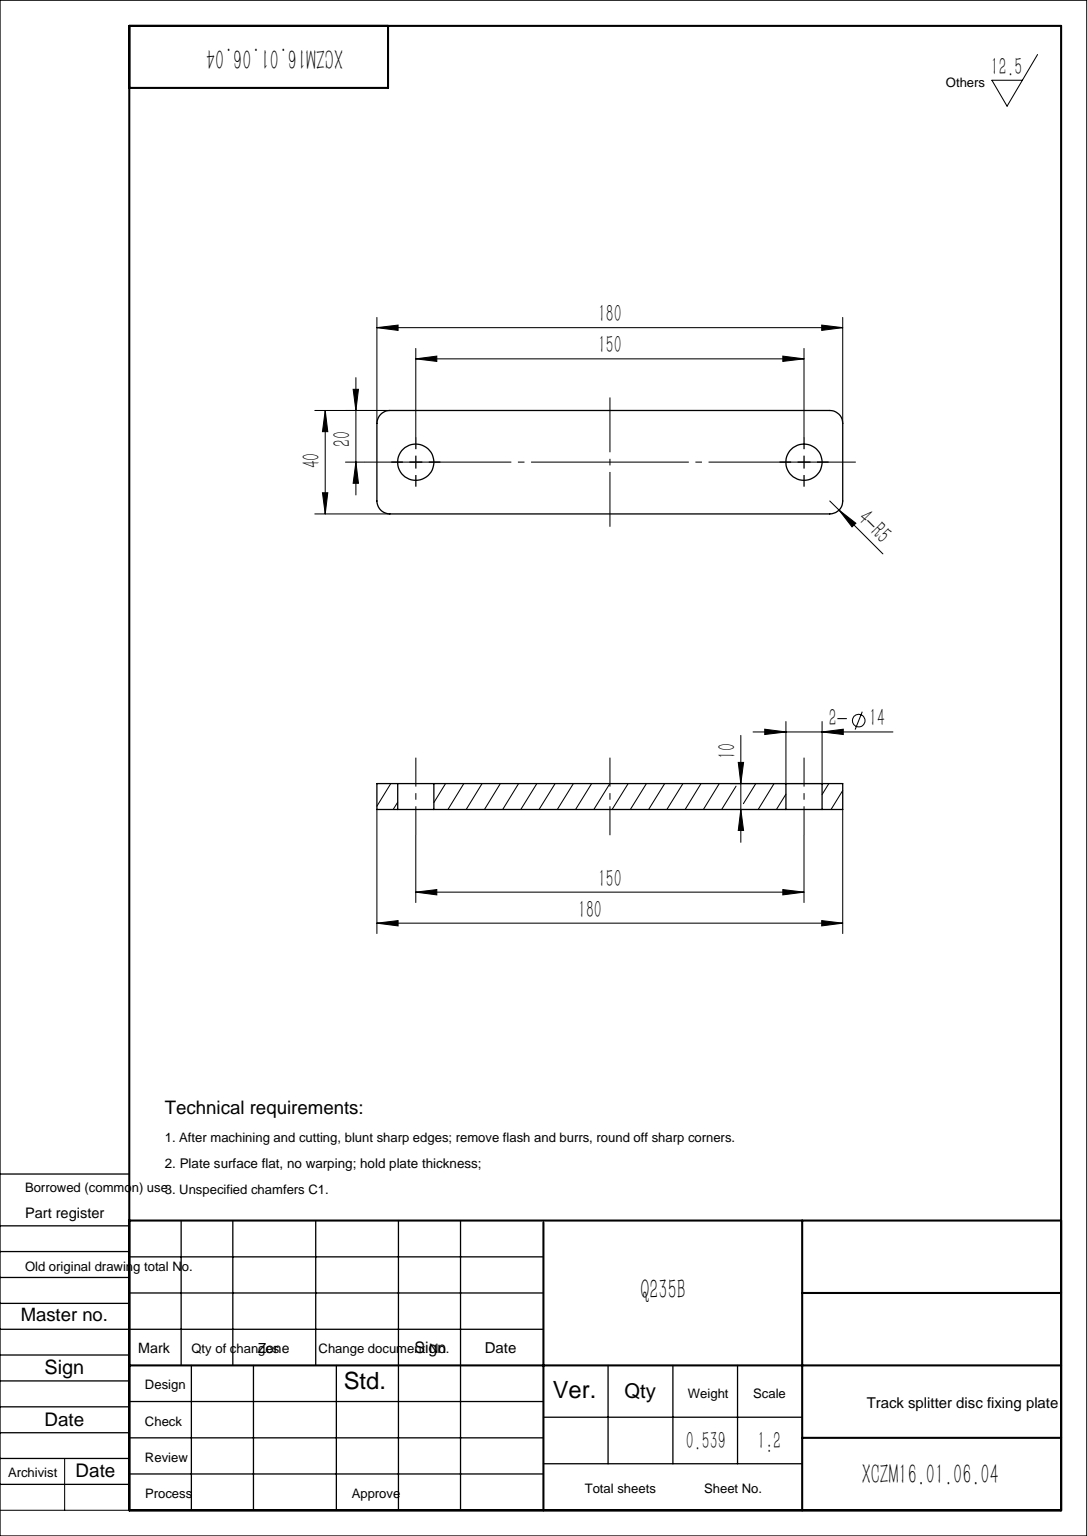
from build123d import *

# Parameters (mm, degrees)
SKETCH2_R           = 7
BOSS_EXTRUDE1_DEPTH = 10


with BuildPart() as part:
    # Sketch2 → Boss-Extrude1 (new body)
    with BuildSketch(Plane(origin=(0, 0, 0), x_dir=(1, 0, 0), z_dir=(0, 1, 0))):
        with BuildLine():
            Line((85, -20), (-85, -20))
            ThreePointArc((-85, -20), (-88.535533906, -18.535533906), (-90, -15))
            Line((-90, -15), (-90, 15))
            ThreePointArc((-90, 15), (-88.535533906, 18.535533906), (-85, 20))
            Line((-85, 20), (85, 20))
            ThreePointArc((85, 20), (88.535533906, 18.535533906), (90, 15))
            Line((90, 15), (90, -15))
            ThreePointArc((90, -15), (88.535533906, -18.535533906), (85, -20))
        make_face()
        with Locations(Location((-75, 0, 0), (0, 0, 270))):
            Circle(SKETCH2_R, mode=Mode.SUBTRACT)
        with Locations(Location((75, 0, 0), (0, 0, 90))):
            Circle(SKETCH2_R, mode=Mode.SUBTRACT)
    extrude(amount=BOSS_EXTRUDE1_DEPTH)


solid = part.part
